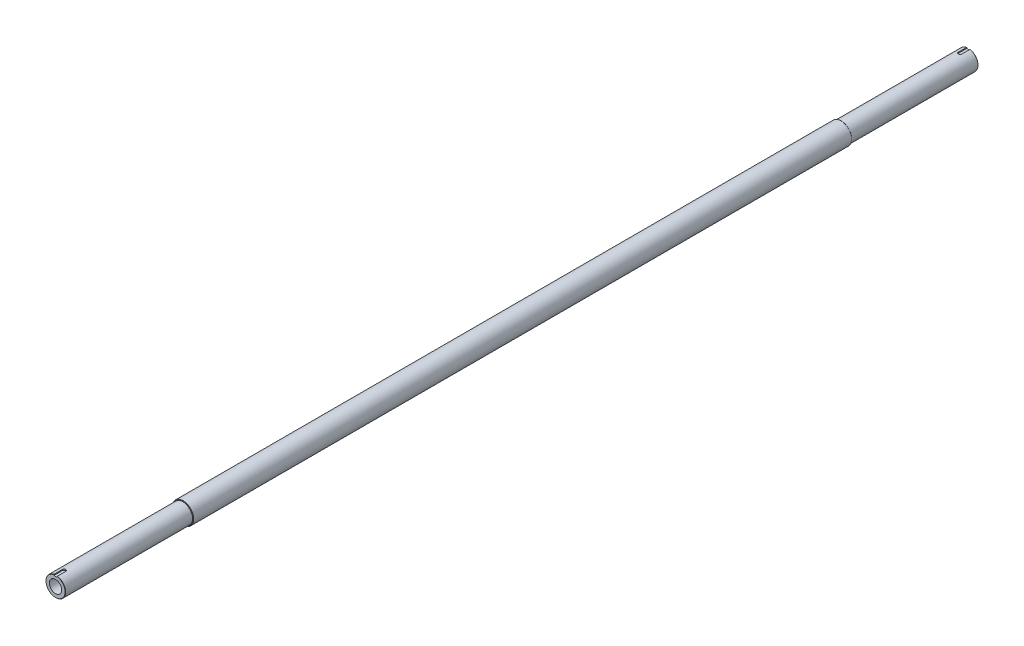
SolidWorks part; units mm, degrees
other "Markup1"
sketch "草图4" plane through (47.5, 47.5, 0) normal (0.0804, 0.6651, -0.7424) x (0.0471, 0.7415, 0.6693)
material "普通碳钢"
ref_plane "Front Plane" through (0, 0, 0) normal (0, 0, 1) x (1, 0, 0)
ref_plane "Top Plane" through (0, 0, 0) normal (0, 1, 0) x (1, 0, 0)
ref_plane "Right Plane" through (0, 0, 0) normal (1, 0, 0) x (0, 0, -1)
other "Configuration Table"
sketch "Sketch1" plane through (0, 0, 0) normal (0, 0, 1) x (1, 0, 0)
  circle A0 centre (0, 0) radius 38
  dimension "D1" = 76
extrude "Boss-Extrude1" add sketch "Sketch1" along normal blind 3254
sketch "Sketch2" plane through (0, 0, 0) normal (0, 0, -1) x (-1, 0, 0)
  circle A0 centre (0, 0) radius 35
  circle A1 centre (0, 0) radius 38
  dimension "D1" = 70
  dimension "D2" = 76
extrude "Cut-Extrude1" cut sketch "Sketch2" against normal blind 453.5
cosmetic thread "Cosmetic Thread3" parameters "D1"=30, "D2"=36
cosmetic thread "Cosmetic Thread4" parameters "D1"=35, "D2"=57.505
sketch "Sketch3" plane through (0, 0, 3254) normal (0, 0, 1) x (1, 0, 0)
  circle A0 centre (0, 0) radius 35
  circle A1 centre (0, 0) radius 38
  dimension "D1" = 70
  dimension "D2" = 76
extrude "Cut-Extrude2" cut sketch "Sketch3" against normal blind 453.5
cosmetic thread "Cosmetic Thread5" parameters "D1"=35, "D2"=57.505
sketch "Sketch5" plane through (0, 0, 0) normal (0, 0, -1) x (-1, 0, 0)
  circle A0 centre (0, 0) radius 22
  dimension "D1" = 44
extrude "Cut-Extrude3" cut sketch "Sketch5" against normal through all
ref_plane "Plane1" through (0, 35, 0) normal (0, 1, 0) x (1, 0, 0)
sketch "Sketch6" plane through (0, 35, 0) normal (0, 1, 0) x (1, 0, 0)
  line L0 (0, 0) -> (0, -30) construction
  line L1 (35, 0) -> (-35, 0) construction
  line L2 (6, 0) -> (6, -30)
  line L3 (-6, 0) -> (-6, -30)
  arc A0 (6, 0) -> (-6, 0) centre (0, 0) ccw
  arc A1 (-6, -30) -> (6, -30) centre (0, -30) ccw
  point P5 (0, -15)
  dimension "D1" = 12
  dimension "D2" = 30
extrude "Cut-Extrude4" cut sketch "Sketch6" against normal blind 4
ref_plane "Plane2" through (0, 0, 1627) normal (0, 0, -1) x (-1, 0, 0)
mirror "Mirror1" about plane through (0, 0, 1627) normal (0, 0, -1) of "Cut-Extrude4"
chamfer "Chamfer1" distance 1 angle 45 4 edges at (0, -35, 3254) (38, 0, 2800.5) (-38, 0, 453.5) (0, -35, 0)
